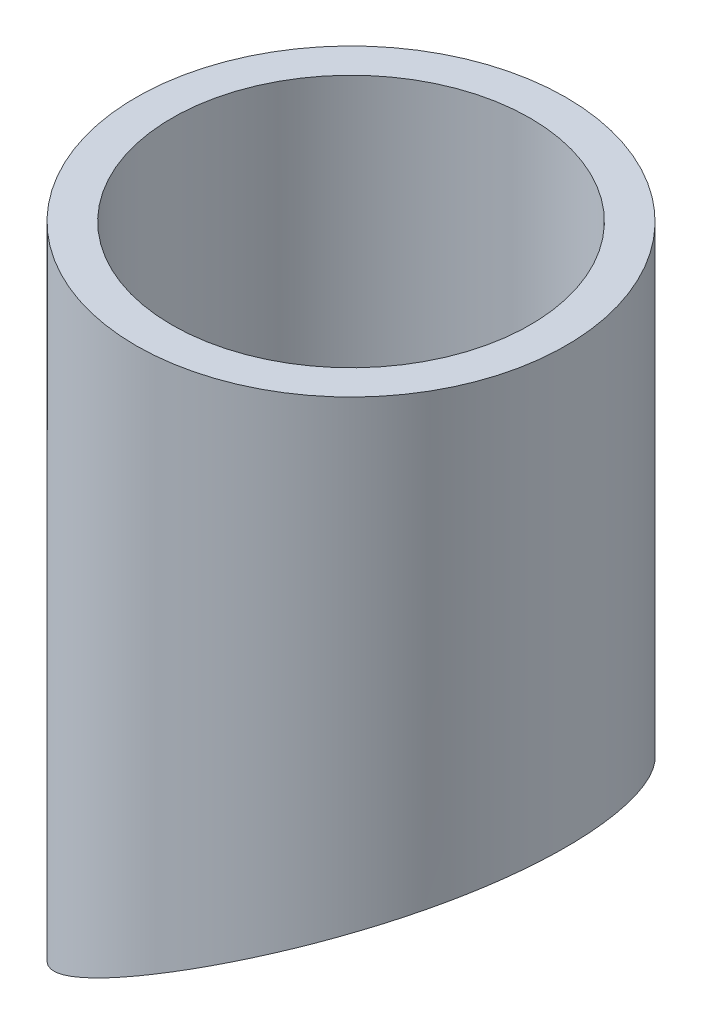
from build123d import *

# Parameters (mm, degrees)
SKETCH2_R               = 30
SKETCH2_R_2             = 25
BOSS_EXTRUDE1_DEPTH     = 300
CUT_EXTRUDE1_DEPTH      = 303.985148151
CUT_EXTRUDE1_DEPTH_BACK = 303.985148151
SKETCH3_R               = 379.5


with BuildPart() as part:
    # Sketch2 → Boss-Extrude1 (new body)
    with BuildSketch(Plane(origin=(0, 0, 0), x_dir=(1, 0, 0), z_dir=(0, 1, 0))):
        with Locations(Location((0, 0, 0), (0, 0, 270))):
            Circle(SKETCH2_R)
        with Locations(Location((0, 0, 0), (0, 0, 270))):
            Circle(SKETCH2_R_2, mode=Mode.SUBTRACT)
    extrude(amount=BOSS_EXTRUDE1_DEPTH)

    # Sketch3 → Cut-Extrude1 (cut, two sides: drawn at the far end of the back side and taken through both)
    with BuildSketch(Plane.XY.offset(-CUT_EXTRUDE1_DEPTH_BACK)):
        with Locations((189.75, -104.83790721)):
            Circle(SKETCH3_R)
    extrude(amount=CUT_EXTRUDE1_DEPTH + CUT_EXTRUDE1_DEPTH_BACK, mode=Mode.SUBTRACT)


solid = part.part
